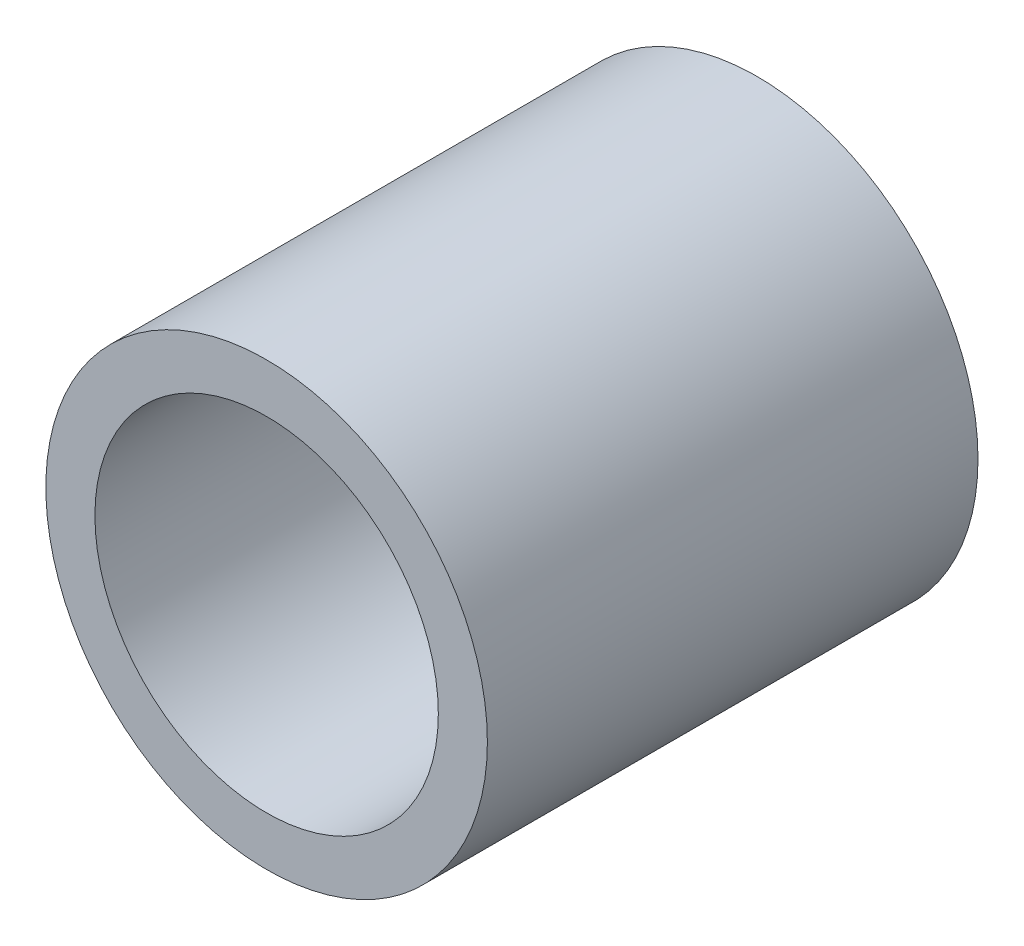
SolidWorks part; units mm, degrees
material "黄铜"
ref_plane "前视基准面" through (0, 0, 0) normal (0, 0, 1) x (1, 0, 0)
ref_plane "上视基准面" through (0, 0, 0) normal (0, 1, 0) x (1, 0, 0)
ref_plane "右视基准面" through (0, 0, 0) normal (1, 0, 0) x (0, 0, -1)
sketch "草图1" plane through (0, 0, 0) normal (0, 0, 1) x (1, 0, 0)
  circle A0 centre (0, 0) radius 20
  circle A1 centre (0, 0) radius 15
  dimension "D1" = 5
extrude "凸台-拉伸1" add sketch "草图1" along normal blind 50
sketch "草图2" plane through (0, 0, 50) normal (0, 0, 1) x (1, 0, 0)
  circle A0 centre (0, 0) radius 22.5
  circle A1 centre (0, 0) radius 20
extrude "凸台-拉伸2" add sketch "草图2" against normal blind 50
sketch "草图3" plane through (0, 0, 50) normal (0, 0, 1) x (1, 0, 0)
  circle A2 centre (0, 0) radius 17.5
  circle A3 centre (0, 0) radius 17.5
  dimension "D1" = 5
extrude "切除-拉伸2" cut sketch "草图3" against normal blind 50
